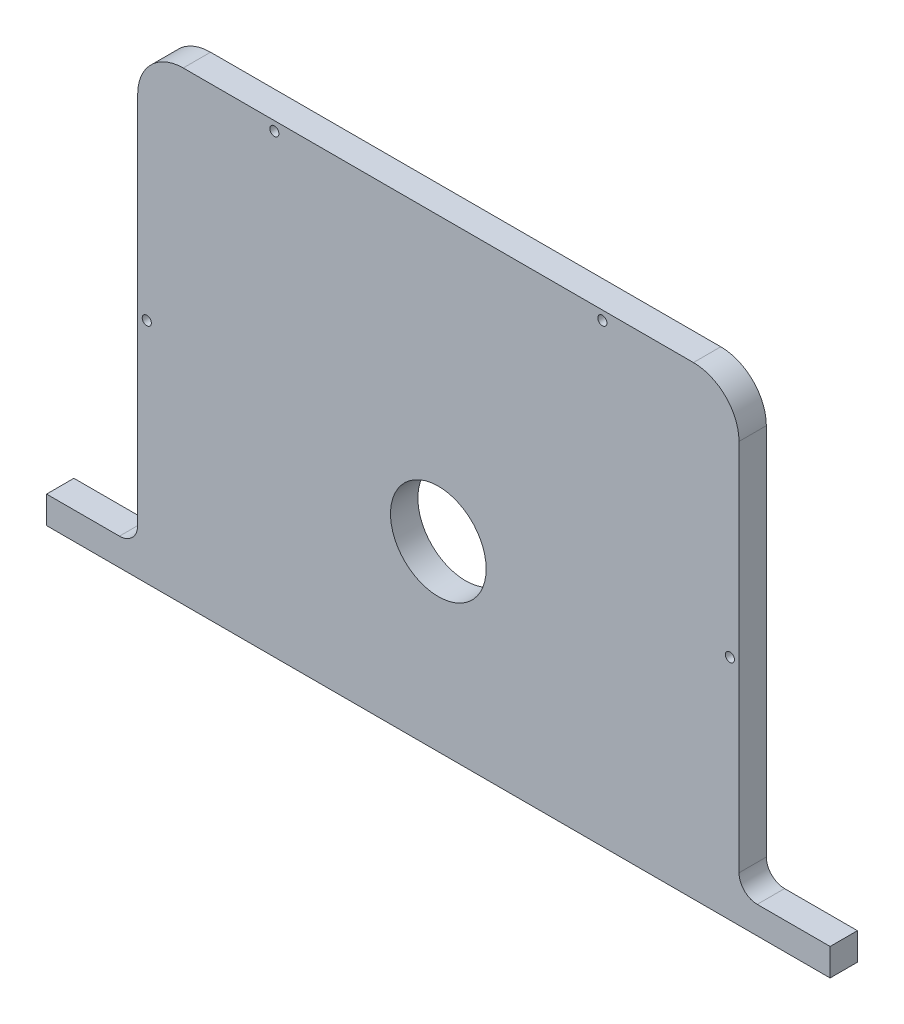
from build123d import *

# Parameters (mm, degrees)
SKETCH1_R           = 5.25
SKETCH1_R_2         = 0.5
BOSS_EXTRUDE1_DEPTH = 3


with BuildPart() as part:
    # Sketch1 → Boss-Extrude1 (new body)
    with BuildSketch(Plane.XY):
        with BuildLine():
            Line((86, 0), (86, 3))
            Line((86, 3), (78, 3))
            ThreePointArc((78, 3), (76.585786438, 3.585786438), (76, 5))
            Line((76, 5), (76, 46))
            ThreePointArc((76, 46), (74.535533906, 49.535533906), (71, 51))
            Line((71, 51), (15, 51))
            ThreePointArc((15, 51), (11.464466094, 49.535533906), (10, 46))
            Line((10, 46), (10, 5))
            ThreePointArc((10, 5), (9.414213562, 3.585786438), (8, 3))
            Line((8, 3), (0, 3))
            Line((0, 3), (0, 0))
            Line((0, 0), (86, 0))
        make_face()
        with Locations((43, 20)):
            Circle(SKETCH1_R, mode=Mode.SUBTRACT)
        with Locations((25, 50)):
            Circle(SKETCH1_R_2, mode=Mode.SUBTRACT)
        with Locations((61, 50)):
            Circle(SKETCH1_R_2, mode=Mode.SUBTRACT)
        with Locations((75, 25)):
            Circle(SKETCH1_R_2, mode=Mode.SUBTRACT)
        with Locations((11, 25)):
            Circle(SKETCH1_R_2, mode=Mode.SUBTRACT)
    extrude(amount=BOSS_EXTRUDE1_DEPTH)


solid = part.part
